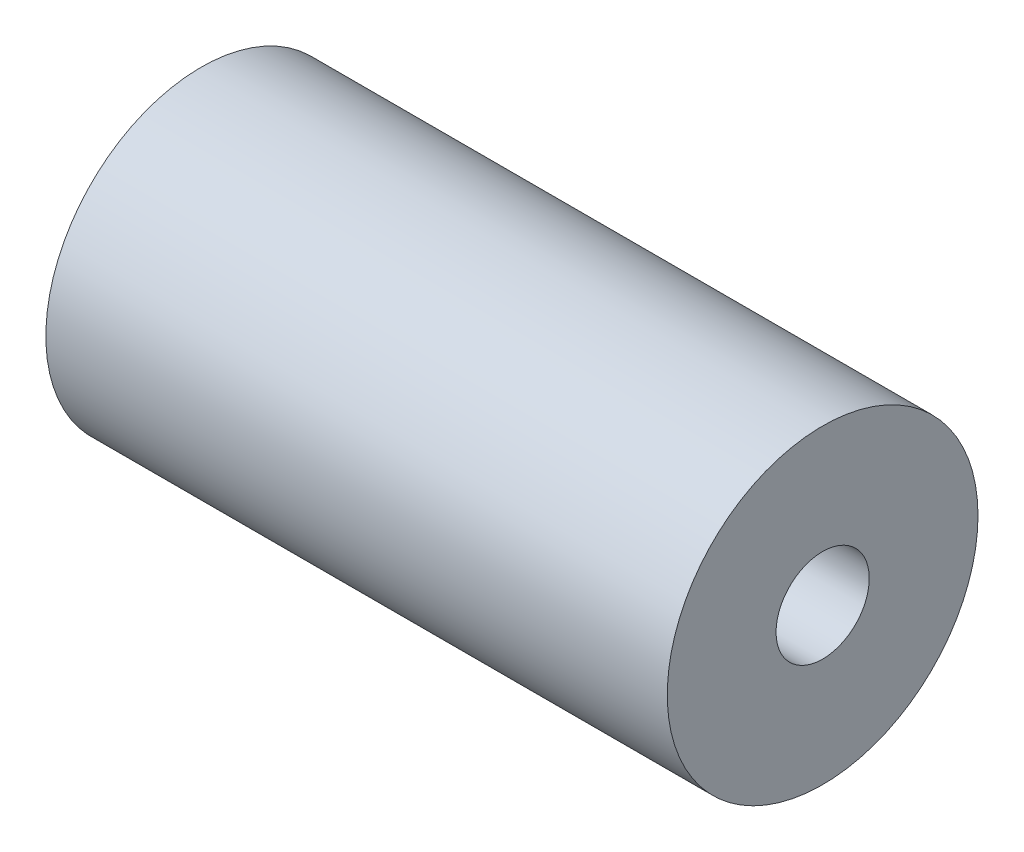
from build123d import *
from build123d.topology import SkipClean

# Parameters (mm, degrees)
SKETCH_1_R      = 10
SKETCH_1_R_2    = 3
EXTRUDE_1_DEPTH = 40
EXTRUDE_START   = 1
SKETCH_3_R      = 7.5
SKETCH_3_R_2    = 3
EXTRUDE_2_DEPTH = 1


with BuildPart() as part:
    # 草图1 → 凸台-拉伸1 (new body)
    with BuildSketch(Plane(origin=(0, 0, 0), x_dir=(0, 0, -1), z_dir=(1, 0, 0))):
        Circle(SKETCH_1_R)
        Circle(SKETCH_1_R_2, mode=Mode.SUBTRACT)
    extrude(amount=EXTRUDE_1_DEPTH)

    # 草图3 → 凸台-拉伸2 (add)
    with SkipClean():  # the faces are left unmerged after this step: merging them gives an invalid solid
        with BuildSketch(Plane.ZY.offset(EXTRUDE_START)):
            with Locations(Location((0, 0, 0), (0, 0, 180))):
                Circle(SKETCH_3_R)
            Circle(SKETCH_3_R_2, mode=Mode.SUBTRACT)
        extrude(amount=-EXTRUDE_2_DEPTH)


solid = part.part
